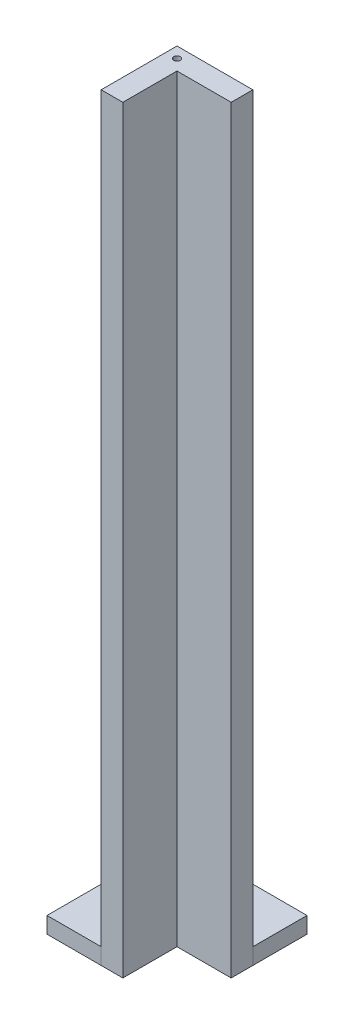
SolidWorks part; units mm, degrees
material "普通碳钢"
ref_plane "Front Plane" through (0, 0, 0) normal (0, 0, 1) x (1, 0, 0)
ref_plane "Top Plane" through (0, 0, 0) normal (0, 1, 0) x (1, 0, 0)
ref_plane "Right Plane" through (0, 0, 0) normal (1, 0, 0) x (0, 0, -1)
sketch "Sketch2" plane through (0, 0, 0) normal (0, 1, 0) x (1, 0, 0)
  line L0 (-10, 60) -> (-10, -60) construction
  line L1 (-60, -60) -> (-10, -60)
  line L2 (-60, -60) -> (-60, 60)
  line L3 (-60, 60) -> (60, 60)
  line L4 (60, 10) -> (60, 60)
  line L5 (-60, -60) -> (60, 60) construction
  line L6 (-60, 60) -> (60, -60) construction
  line L7 (-71.74, 10) -> (86.888, 10) construction
  line L8 (-10, -60) -> (-10, 10)
  line L9 (-10, 10) -> (60, 10)
  line L10 (-35, -60) -> (-35, 48.2507) construction
  circle A0 centre (-35, -10) radius 8
  circle A1 centre (10, 35) radius 8
  point P0 (0, 0)
  dimension "D6" = 16
  dimension "D7" = 25
  dimension "D1" = 120
  dimension "D2" = 120
  dimension "D3" = 50
  dimension "D4" = 50
  dimension "D5" = 70
  dimension "D8" = 70
extrude "Boss-Extrude1" add sketch "Sketch2" along normal blind 15
sketch "Sketch3" plane through (0, 15, 0) normal (0, 1, 0) x (1, 0, 0)
  line L0 (-10, -60) -> (-10, 10) construction
  line L1 (-10, 10) -> (60, 10) construction
  line L2 (-10, -60) -> (-10, 10)
  line L3 (-10, 10) -> (60, 10)
  line L4 (-10, -60) -> (10, -60)
  line L5 (60, 10) -> (60, -10)
  line L6 (10, -60) -> (10, -10)
  line L7 (10, -10) -> (60, -10)
  dimension "D1" = 20
  dimension "D2" = 20
extrude "Boss-Extrude2" add sketch "Sketch3" against normal blind 15 and the other way blind 685 separate body
sketch "Sketch4" plane through (0, 700, 0) normal (0, 1, 0) x (1, 0, 0)
  line L0 (60, 0) -> (-18.1817, 0) construction
  line L1 (60, -10) -> (60, 10) construction
  line L2 (0, -60) -> (0, 29.6461) construction
  line L3 (-10, -60) -> (10, -60) construction
  circle A0 centre (0, 0) radius 3
extrude "Cut-Extrude1" cut sketch "Sketch4" against normal blind 20
